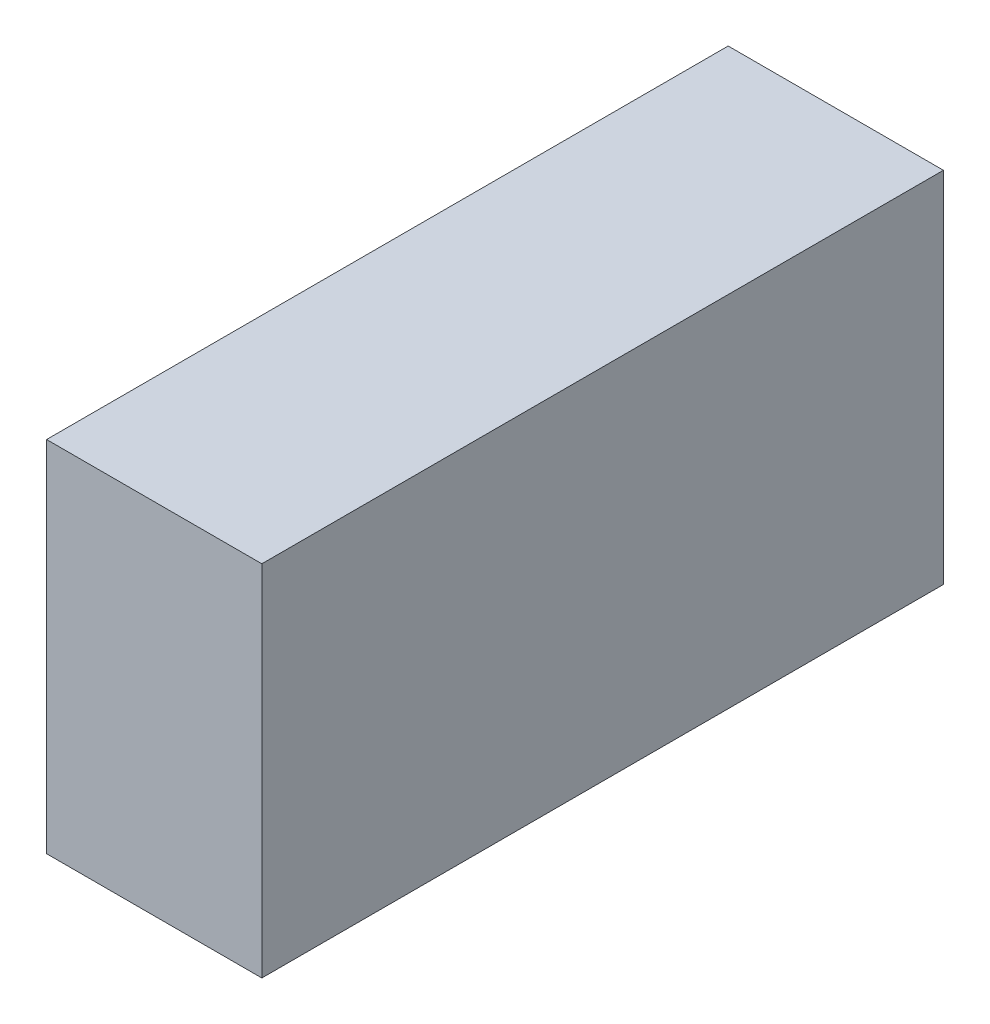
SolidWorks part; units mm, degrees
ref_plane "Front Plane" through (0, 0, 0) normal (0, 0, 1) x (1, 0, 0)
ref_plane "Top Plane" through (0, 0, 0) normal (0, 1, 0) x (1, 0, 0)
ref_plane "Right Plane" through (0, 0, 0) normal (1, 0, 0) x (0, 0, -1)
sketch "Sketch1" plane through (0, 0, 0) normal (1, 0, 0) x (0, 0, -1)
  line L1 (0, 0) -> (38, 0)
  line L2 (0, 0) -> (0, 20)
  line L3 (0, 20) -> (38, 20)
  line L4 (38, 0) -> (38, 20)
  dimension "D1" = 38
  dimension "D2" = 20
extrude "Boss-Extrude1" add sketch "Sketch1" along normal blind 12
